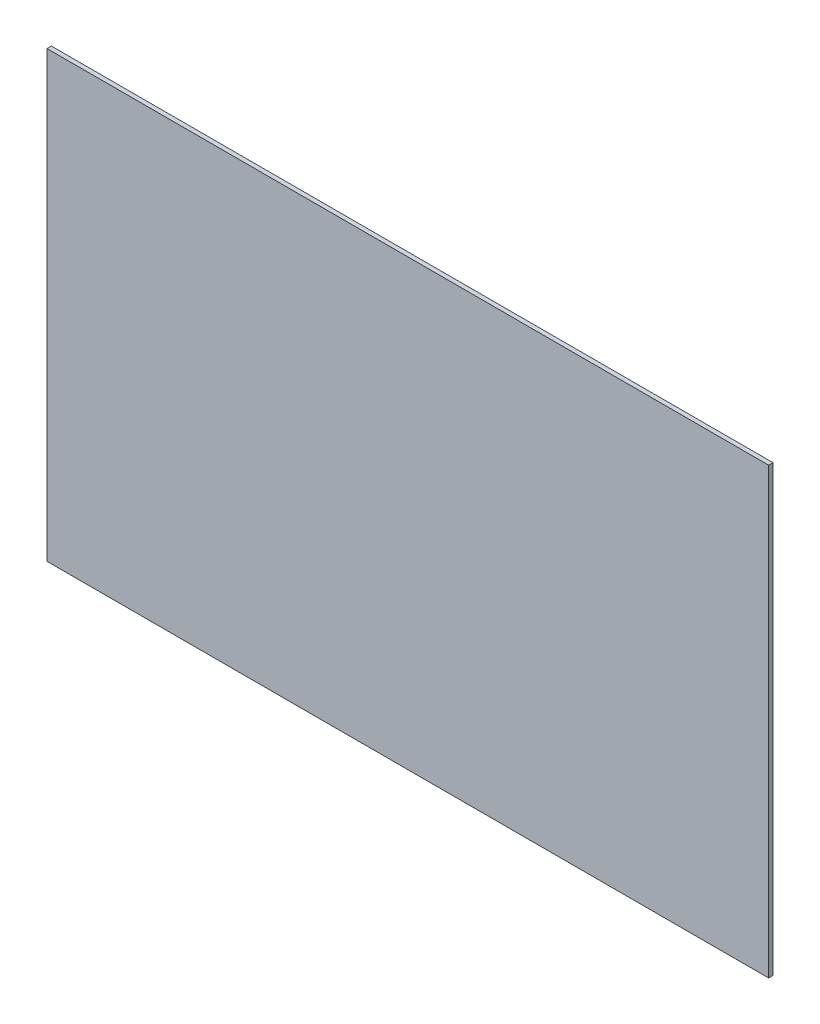
SolidWorks part; units mm, degrees
material "普通碳钢"
ref_plane "Front Plane" through (0, 0, 0) normal (0, 0, 1) x (1, 0, 0)
ref_plane "Top Plane" through (0, 0, 0) normal (0, 1, 0) x (1, 0, 0)
ref_plane "Right Plane" through (0, 0, 0) normal (1, 0, 0) x (0, 0, -1)
sketch "Sketch1" plane through (0, 0, 0) normal (0, 0, 1) x (1, 0, 0)
  line L1 (-165.1, 101.6) -> (165.1, 101.6)
  line L2 (-165.1, 101.6) -> (-165.1, -101.6)
  line L3 (-165.1, -101.6) -> (165.1, -101.6)
  line L4 (165.1, 101.6) -> (165.1, -101.6)
  dimension "D1" = 330.2
  dimension "D2" = 203.2
  dimension "D3" = 165.1
  dimension "D4" = 101.6
extrude "Boss-Extrude1" add sketch "Sketch1" along normal mid plane 2
